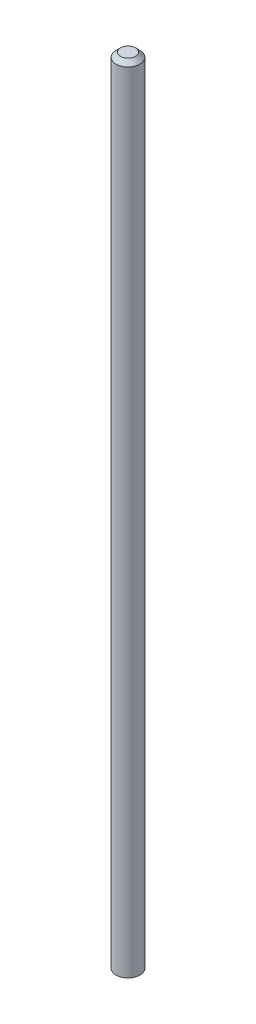
SolidWorks part; units mm, degrees
ref_plane "Front Plane" through (0, 0, 0) normal (0, 0, 1) x (1, 0, 0)
ref_plane "Top Plane" through (0, 0, 0) normal (0, 1, 0) x (1, 0, 0)
ref_plane "Right Plane" through (0, 0, 0) normal (1, 0, 0) x (0, 0, -1)
sketch "Sketch1" plane through (0, 0, 0) normal (0, 1, 0) x (1, 0, 0)
  circle A0 centre (0, 0) radius 8
  dimension "D1" = 16
extrude "Boss-Extrude1" add sketch "Sketch1" along normal blind 531.5
cosmetic thread "Cosmetic Thread1" parameters "D1"=30, "D2"=14
cosmetic thread "Cosmetic Thread2" parameters "D1"=30, "D2"=14
chamfer "Chamfer1" distance 3 angle 45 1 edges at (0, 531.5, 8)
